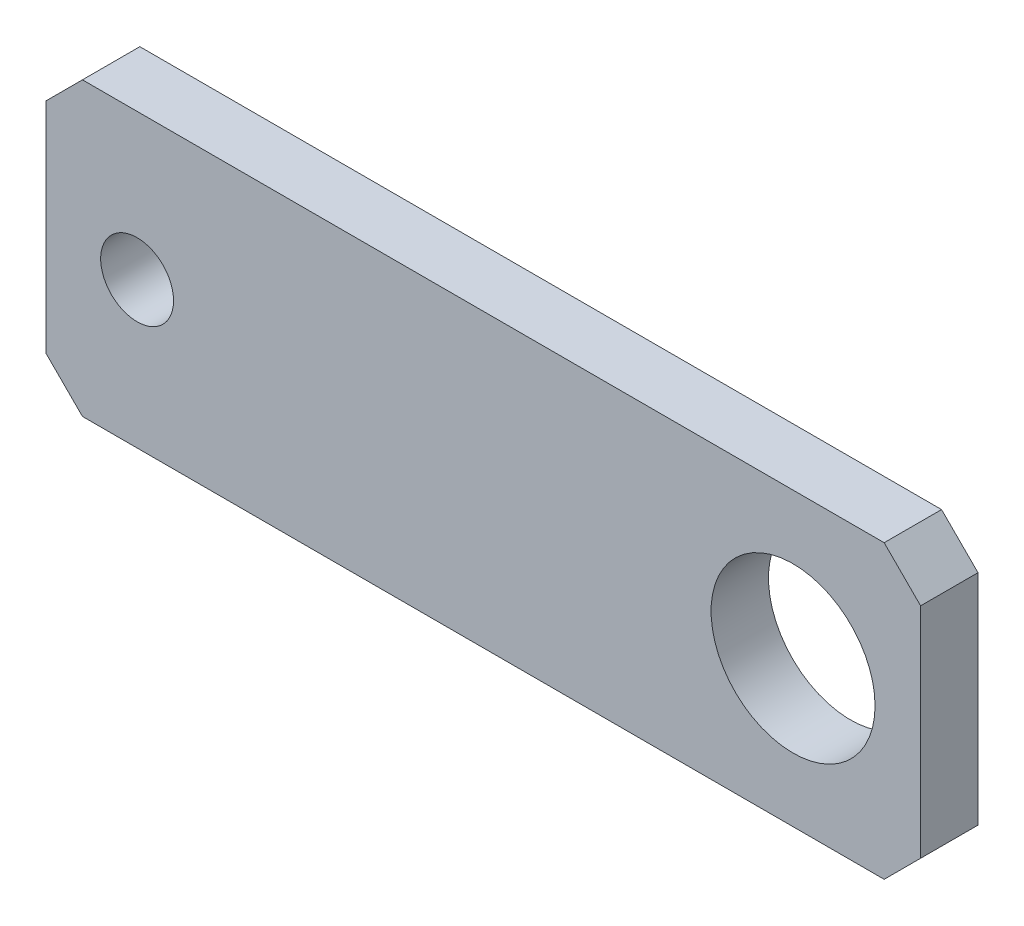
from build123d import *

# Parameters (mm, degrees)
SKETCH1_W      = 152.4
SKETCH1_H      = 50.8
SKETCH1_R      = 14.2875
SKETCH1_R_2    = 6.35
EXTRUDE1_DEPTH = 5
CHAMFER1_SIZE  = 6.35


with BuildPart() as part:
    # Sketch1 → Extrude1 (new, symmetric)
    with BuildSketch(Plane.XY):
        with Locations((3.175, 0)):
            Rectangle(SKETCH1_W, SKETCH1_H)
        with Locations((57.15, 0)):
            Circle(SKETCH1_R, mode=Mode.SUBTRACT)
        with Locations((-57.15, 0)):
            Circle(SKETCH1_R_2, mode=Mode.SUBTRACT)
    extrude(amount=EXTRUDE1_DEPTH, both=True)

    # Chamfer1
    chamfer1_edges = [part.edges().sort_by_distance(p)[0] for p in [
        (-73.025, 25.4, 0),
        (79.375, 25.4, 0),
        (79.375, -25.4, 0),
        (-73.025, -25.4, 0),
    ]]
    chamfer(chamfer1_edges, length=CHAMFER1_SIZE)


solid = part.part
